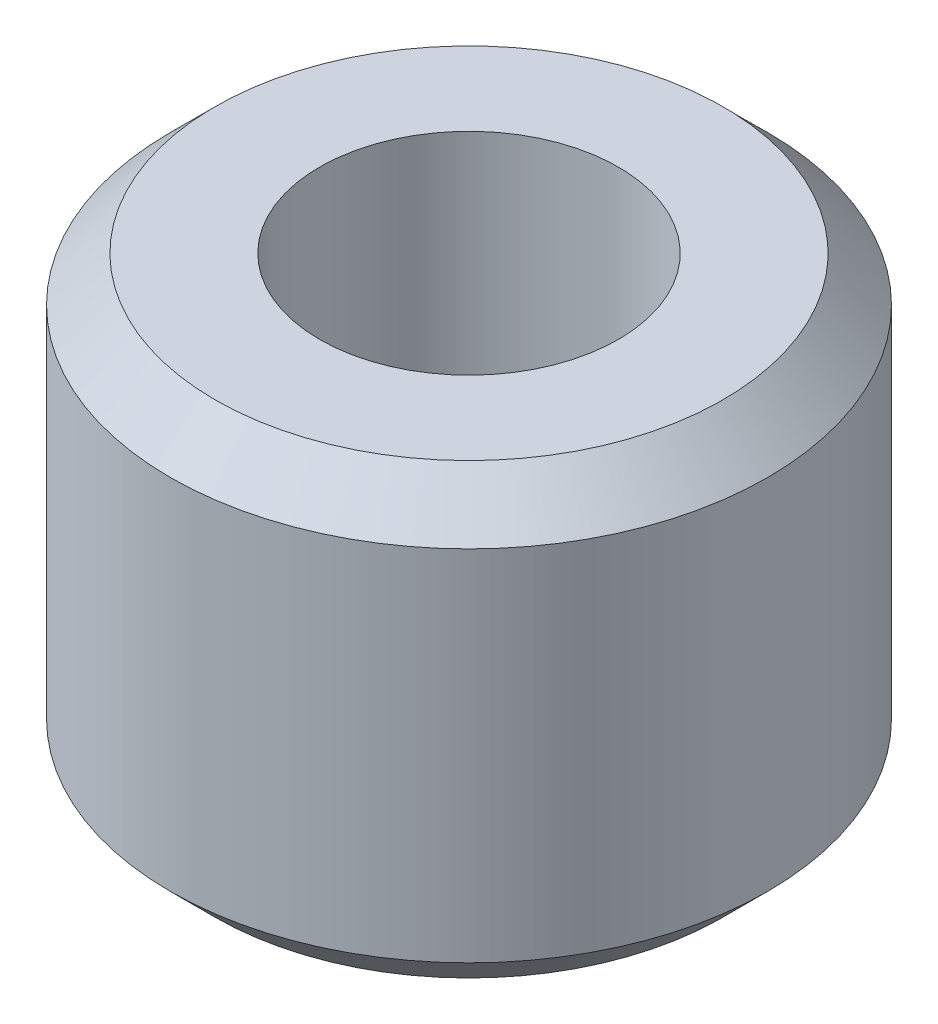
SolidWorks part; units mm, degrees
material "20 steel"
ref_plane "Front Plane" through (0, 0, 0) normal (0, 0, 1) x (1, 0, 0)
ref_plane "Top Plane" through (0, 0, 0) normal (0, 1, 0) x (1, 0, 0)
ref_plane "Right Plane" through (0, 0, 0) normal (1, 0, 0) x (0, 0, -1)
sketch "Sketch1" plane through (0, 0, 0) normal (0, 1, 0) x (1, 0, 0)
  circle A0 centre (0, 0) radius 20
  circle A1 centre (0, 0) radius 10
  dimension "D1" = 40
  dimension "D2" = 20
extrude "Boss-Extrude1" add sketch "Sketch1" along normal blind 30
chamfer "Chamfer1" distance 3 angle 45 2 edges at (0, 0, 20) (0, 30, 20)
